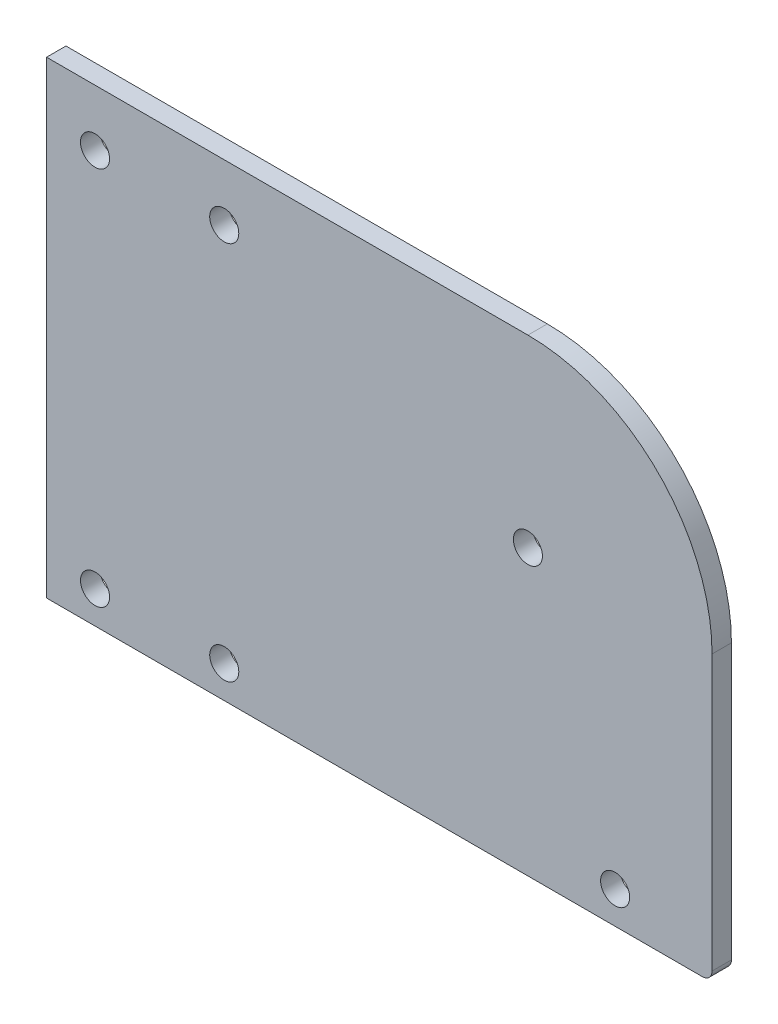
SolidWorks part; units mm, degrees
material "普通碳钢"
ref_plane "前视基准面" through (0, 0, 0) normal (0, 0, 1) x (1, 0, 0)
ref_plane "上视基准面" through (0, 0, 0) normal (0, 1, 0) x (1, 0, 0)
ref_plane "右视基准面" through (0, 0, 0) normal (1, 0, 0) x (0, 0, -1)
sketch "草图1" plane through (0, 0, 0) normal (0, 0, 1) x (1, 0, 0)
  line L0 (0, 72.5) -> (0, 0) construction
  line L1 (-103, 72.5) -> (103, 72.5)
  line L2 (-103, 72.5) -> (-103, -72.5)
  line L3 (-103, -72.5) -> (103, -72.5)
  line L4 (103, 72.5) -> (103, -72.5)
  line L5 (0, 0) -> (103, 0) construction
  dimension "D1" = 206
  dimension "D2" = 145
extrude "凸台-拉伸1" add sketch "草图1" along normal blind 6
sketch "草图2" plane through (0, 0, 6) normal (0, 0, 1) x (1, 0, 0)
  line L0 (103, 72.5) -> (-103, 72.5) construction
  line L1 (-103, -72.5) -> (-3, -72.5)
  line L2 (-103, -72.5) -> (-103, -7.5)
  line L3 (-103, -7.5) -> (-3, -7.5)
  line L4 (-3, -72.5) -> (-3, -7.5)
  dimension "D1" = 80
  dimension "D2" = 100
extrude "切除-拉伸1" [suppressed] cut sketch "草图2" against normal through all
sketch "草图3" plane through (0, 0, 6) normal (0, 0, 1) x (1, 0, 0)
  line L0 (103, 72.5) -> (-103, 72.5) construction
  line L1 (-103, 72.5) -> (-103, -72.5) construction
  circle A0 centre (-88, 55) radius 4.5
  circle A1 centre (-48, 55) radius 4.5
  circle A2 centre (-88, -62.5) radius 4.5
  circle A3 centre (-48, -62.5) radius 4.5
  dimension "D1" = 9
  dimension "D2" = 40
  dimension "D3" = 117.5
  dimension "D4" = 17.5
  dimension "D5" = 15
extrude "切除-拉伸2" cut sketch "草图3" against normal through all
sketch "草图4" plane through (0, 0, 6) normal (0, 0, 1) x (1, 0, 0)
  line L0 (103, 72.5) -> (-103, 72.5) construction
  line L1 (-103, 72.5) -> (-103, -72.5) construction
  circle A0 centre (46, 15.5) radius 4.5
  dimension "D1" = 9
  dimension "D2" = 57
  dimension "D3" = 149
extrude "切除-拉伸3" cut sketch "草图4" against normal through all
fillet "圆角1" [suppressed] radius 57
fillet "圆角2" [suppressed] radius 10
fillet "圆角3" [suppressed] radius 10
fillet "圆角4" radius 57 1 edges at (103, 72.5, 3)
sketch "草图5" plane through (0, 0, 6) normal (0, 0, 1) x (1, 0, 0)
  line L0 (46, 72.5) -> (-103, 72.5) construction
  line L1 (103, -72.5) -> (103, 15.5) construction
  circle A0 centre (88, 61) radius 2.75
  dimension "D1" = 11.5
  dimension "D2" = 15
  dimension "D3" = 5.5
extrude "切除-拉伸4" [suppressed] cut sketch "草图5" against normal through all
sketch "草图6" plane through (0, 0, 0) normal (0, 0, 1) x (1, 0, 0)
  line L0 (-88, 55) -> (-48, 55) construction
  line L1 (-73, 35) -> (-63, 35)
  line L2 (-73, 35) -> (-73, -35)
  line L3 (-73, -35) -> (-63, -35)
  line L4 (-63, 35) -> (-63, -35)
  line L5 (-68, 55) -> (-68, -39.8746) construction
  line L6 (-103, 0) -> (-46.6746, 0) construction
  line L7 (-103, 72.5) -> (-103, -72.5) construction
  dimension "D1" = 10
  dimension "D2" = 70
extrude "凸台-拉伸2" [suppressed] add sketch "草图6" against normal blind 22
chamfer "倒角1" [suppressed] distance 5 angle 45
sketch "草图7" plane through (0, 0, 0) normal (0, 0, -1) x (-1, 0, 0)
  line L1 (-103, -72.5) -> (-98, -72.5)
  line L2 (-103, -72.5) -> (-103, -27.5)
  line L3 (-103, -27.5) -> (-98, -27.5)
  line L4 (-98, -72.5) -> (-98, -27.5)
  dimension "D1" = 5
  dimension "D2" = 45
extrude "切除-拉伸5" [suppressed] cut sketch "草图7" against normal blind 10
hole_wizard "M4 螺纹孔1" positions "草图9" profile "草图8" tap size "M4" standard "Iso"
sketch "草图9" [suppressed] plane through (98, 0, 0) normal (1, 0, 0) x (0, 0, -1)
  line L0 (-4, -72.5) -> (-4, -26.1551) construction
  line L1 (-8, -72.5) -> (0, -72.5) construction
  point P0 (-4, -62.5)
  point P2 (-4, -37.5)
  dimension "D1" = 10
  dimension "D2" = 25
sketch "草图8" plane through (98, -62.5, 4) normal (0, 1, 0) x (0, 0, -1)
  line L0 (0, 0) -> (0, 12.4914)
  line L1 (0, 12.4914) -> (1.65, 11.5)
  line L2 (1.65, 11.5) -> (1.65, 0)
  line L5 (1.65, 0) -> (0, 0)
  line L10 (0, 12.4914) -> (-1.65, 11.5) construction
  line L11 (0, -6.35) -> (0, 107.95) construction
  dimension "螺纹孔钻头直径" = 3.3
  dimension "螺纹孔钻头深度" = 11.5
  dimension "导头角度" = 118
cosmetic thread "孔螺蚊线1" [suppressed] parameters "D1"=8, "D2"=4
cosmetic thread "孔螺蚊线2" [suppressed] parameters "D1"=8, "D2"=4
fillet "圆角5" [suppressed] radius 3
sketch "草图10" plane through (0, 0, 0) normal (0, 0, -1) x (-1, 0, 0)
  line L0 (103, -72.5) -> (-103, -72.5) construction
  line L1 (-103, -72.5) -> (-103, 15.5) construction
  circle A0 centre (-73, -62.5) radius 4.5
  dimension "D1" = 9
  dimension "D2" = 10
  dimension "D3" = 30
extrude "切除-拉伸6" cut sketch "草图10" against normal blind 10
fillet "圆角6" radius 3 1 edges at (103, -72.5, 3)
